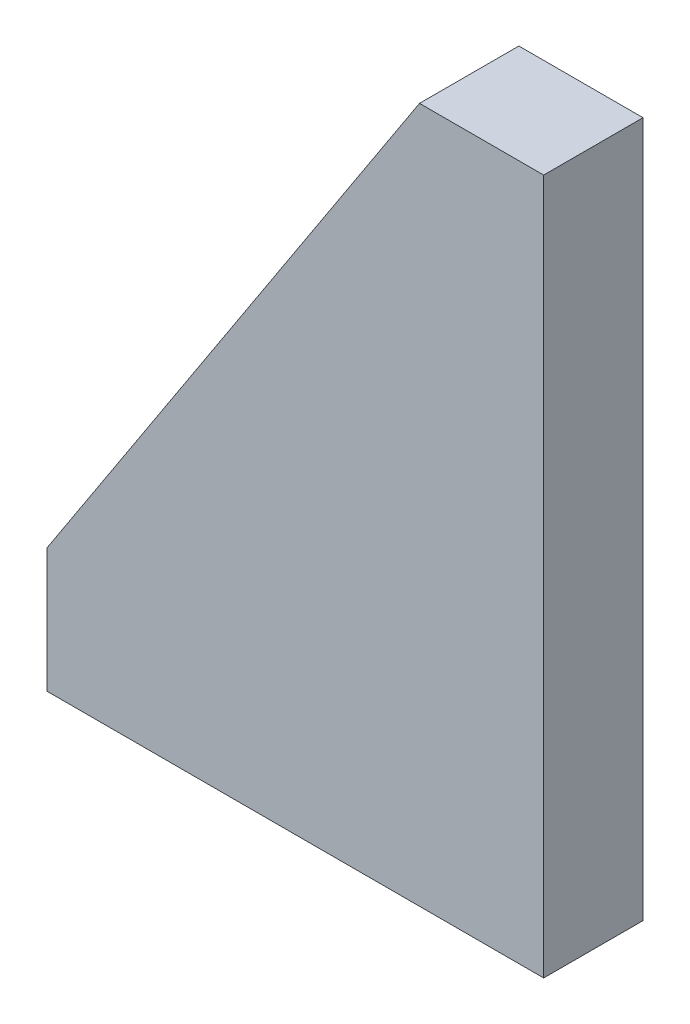
SolidWorks part; units mm, degrees
material "Q235"
ref_plane "Front Plane" through (0, 0, 0) normal (0, 0, 1) x (1, 0, 0)
ref_plane "Top Plane" through (0, 0, 0) normal (0, 1, 0) x (1, 0, 0)
ref_plane "Right Plane" through (0, 0, 0) normal (1, 0, 0) x (0, 0, -1)
sketch "Sketch1" plane through (0, 0, 0) normal (0, 0, 1) x (1, 0, 0)
  line L0 (0, 0) -> (100, 0)
  line L1 (100, 0) -> (100, 140)
  line L2 (100, 140) -> (75, 140)
  line L3 (75, 140) -> (0, 25)
  line L4 (0, 25) -> (0, 0)
  dimension "D1" = 100
  dimension "D2" = 140
  dimension "D3" = 25
  dimension "D4" = 25
extrude "Boss-Extrude1" add sketch "Sketch1" along normal blind 20
